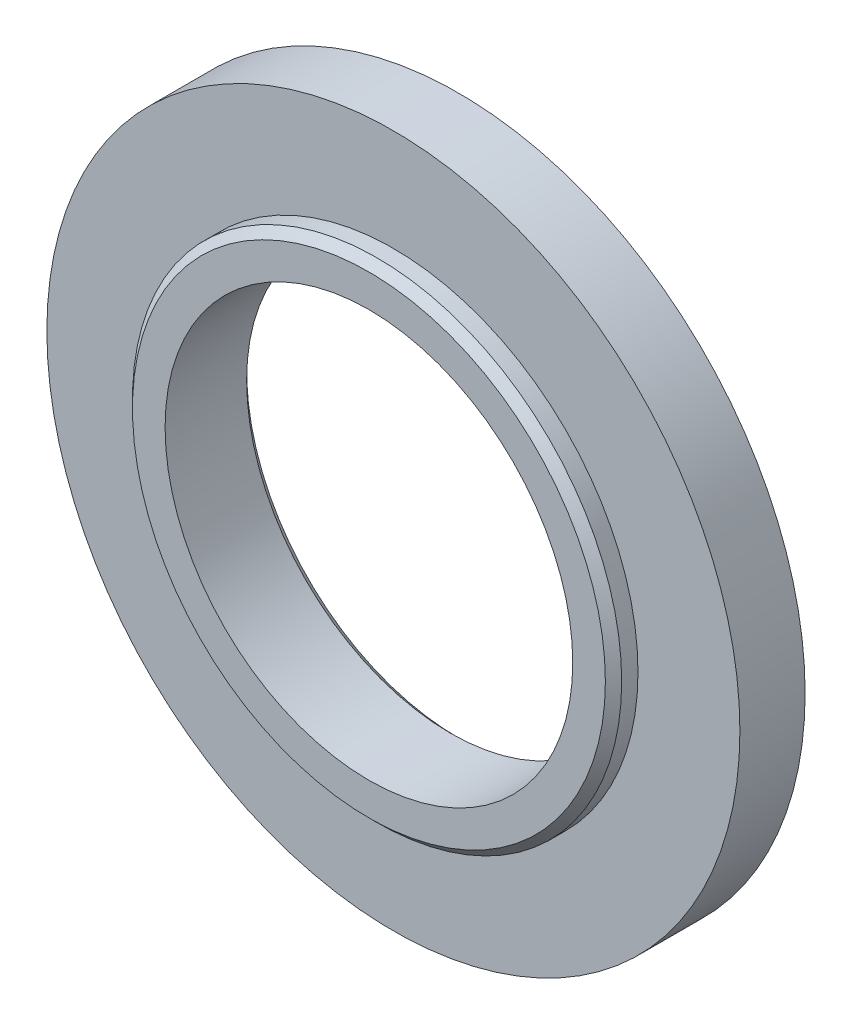
from build123d import *

# Parameters (mm, degrees)
SKETCH1_R             = 42.5
SKETCH1_R_2           = 25
BOSS_EXTRUDE1_DEPTH   = 8
SKETCH2_R             = 30
SKETCH2_R_2           = 25
BOSS_EXTRUDE2_DEPTH   = 3
CHAMFER1_SIZE         = 1
M4_TAPPED_HOLE1_D     = 3.3
M4_TAPPED_HOLE1_DEPTH = 6
M4_TAPPED_HOLE1_TIP   = 0.991420021


with BuildPart() as part:
    # Sketch1 → Boss-Extrude1 (new body)
    with BuildSketch(Plane.XY):
        Circle(SKETCH1_R)
        Circle(SKETCH1_R_2, mode=Mode.SUBTRACT)
    extrude(amount=BOSS_EXTRUDE1_DEPTH)

    # Sketch2 → Boss-Extrude2 (add)
    with BuildSketch(Plane.XY.offset(8)):
        Circle(SKETCH2_R)
        Circle(SKETCH2_R_2, mode=Mode.SUBTRACT)
    extrude(amount=BOSS_EXTRUDE2_DEPTH)

    # Chamfer1
    chamfer1_edges = [part.edges().sort_by_distance(p)[0] for p in [
        (-30, 0, 11),
        (-25, 0, 0),
    ]]
    chamfer(chamfer1_edges, length=CHAMFER1_SIZE)

    # M4 Tapped Hole1
    with Locations(Plane(origin=(18.5, 32.04293994, 0), x_dir=(-1, 0, 0), z_dir=(0, 0, -1))):
        with Locations((0, 0), (37, 0), (55.5, -32.04293994), (37, -64.08587988), (0, -64.08587988), (-18.5, -32.04293994)):
            Hole(M4_TAPPED_HOLE1_D / 2, depth=M4_TAPPED_HOLE1_DEPTH)
            with Locations((0, 0, -(M4_TAPPED_HOLE1_DEPTH + M4_TAPPED_HOLE1_TIP / 2))):  # 118° drill point
                Cone(0, M4_TAPPED_HOLE1_D / 2, M4_TAPPED_HOLE1_TIP, mode=Mode.SUBTRACT)


solid = part.part
